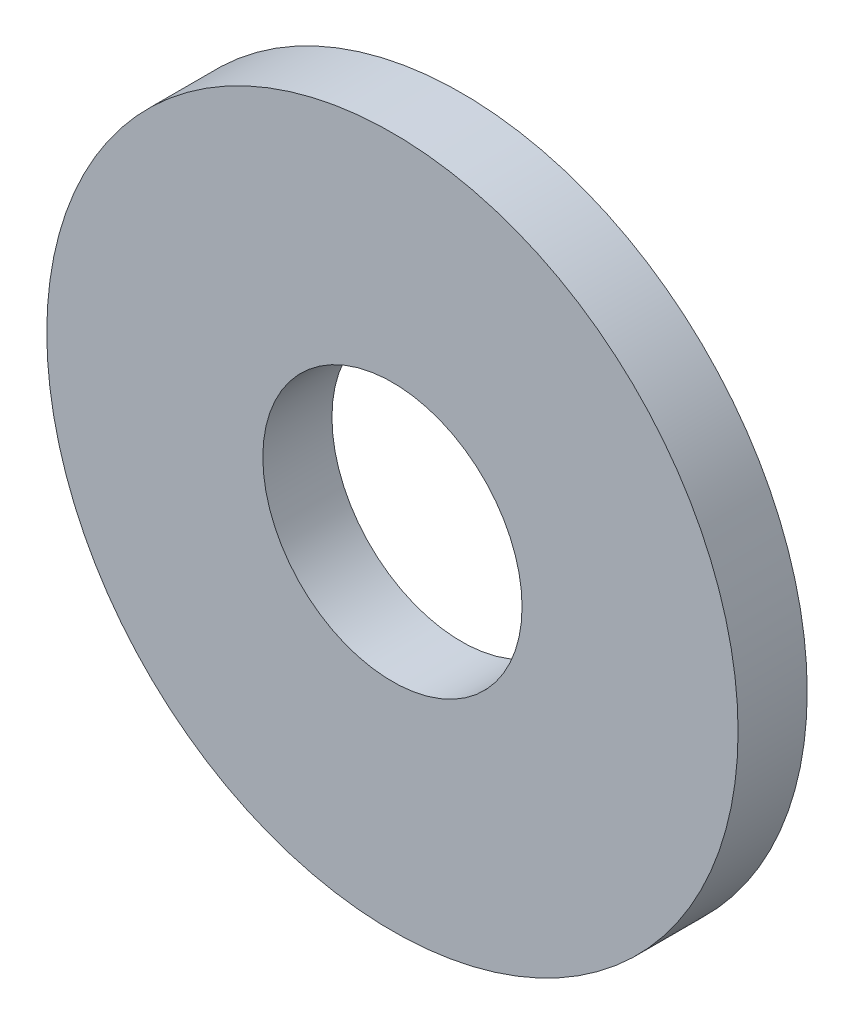
SolidWorks part; units mm, degrees
ref_plane "Front Plane" through (0, 0, 0) normal (0, 0, 1) x (1, 0, 0)
ref_plane "Top Plane" through (0, 0, 0) normal (0, 1, 0) x (1, 0, 0)
ref_plane "Right Plane" through (0, 0, 0) normal (1, 0, 0) x (0, 0, -1)
sketch "Sketch1" plane through (0, 0, 0) normal (0, 0, 1) x (1, 0, 0)
  circle A0 centre (0, 0) radius 7.5
  circle A1 centre (0, 0) radius 20
  dimension "D1" = 15
  dimension "D2" = 40
extrude "Boss-Extrude1" add sketch "Sketch1" along normal blind 4
